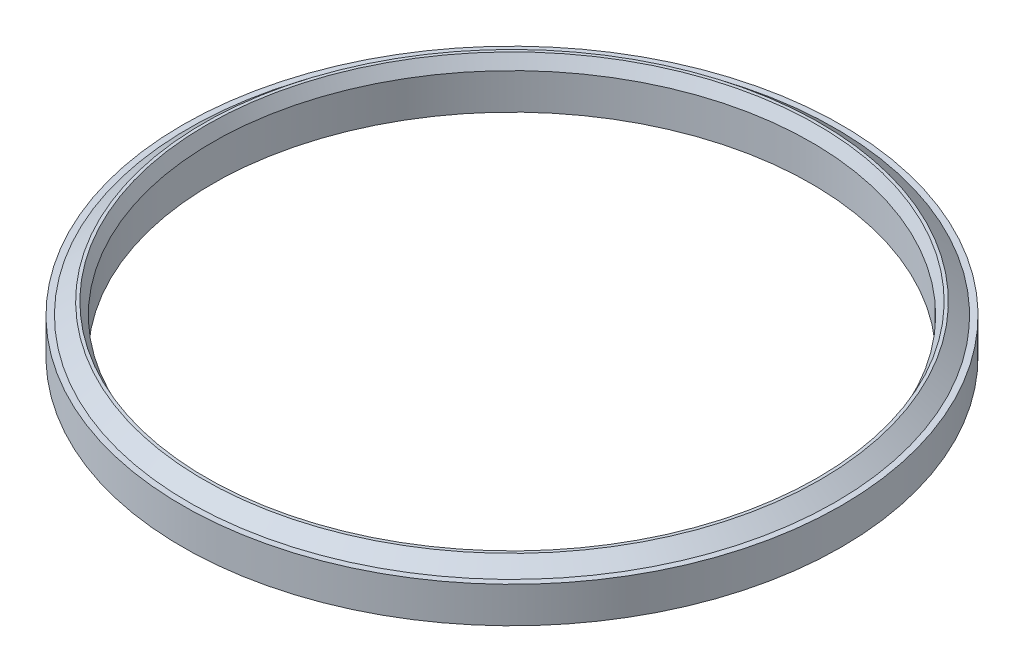
from build123d import *


with BuildPart() as part:
    # Sketch2 → Revolve1 (revolve)
    with BuildSketch(Plane.XY):
        Polygon((50, 0), (55, 0), (55, 6), (54, 6), (51.5, 8), (51, 8), (50, 6), align=None)
    revolve(axis=Axis((0, -1000, 0), (0, 1, 0)))


solid = part.part
